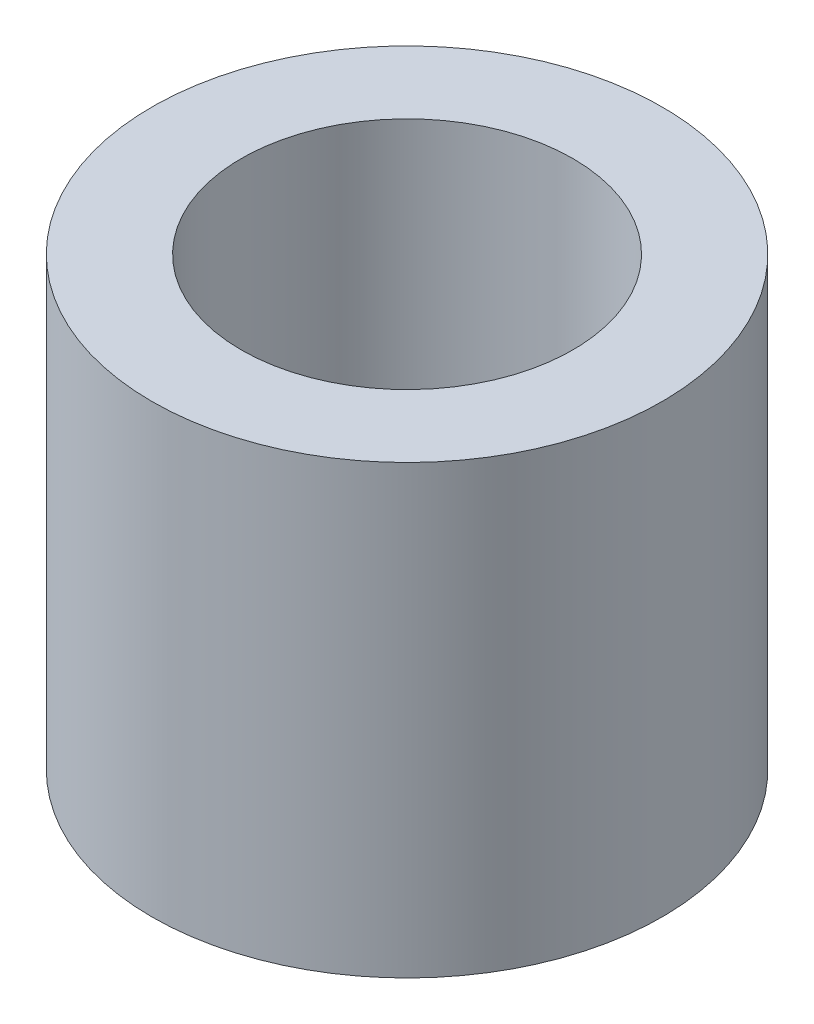
SolidWorks part; units mm, degrees
ref_plane "Front Plane" through (0, 0, 0) normal (0, 0, 1) x (1, 0, 0)
ref_plane "Top Plane" through (0, 0, 0) normal (0, 1, 0) x (1, 0, 0)
ref_plane "Right Plane" through (0, 0, 0) normal (1, 0, 0) x (0, 0, -1)
sketch "Sketch1" plane through (0, 0, 0) normal (0, 1, 0) x (1, 0, 0)
  circle A0 centre (0, 0) radius 2.6
  circle A1 centre (0, 0) radius 4
  dimension "D1" = 5.2
  dimension "D2" = 8
extrude "Boss-Extrude1" add sketch "Sketch1" along normal blind 7
